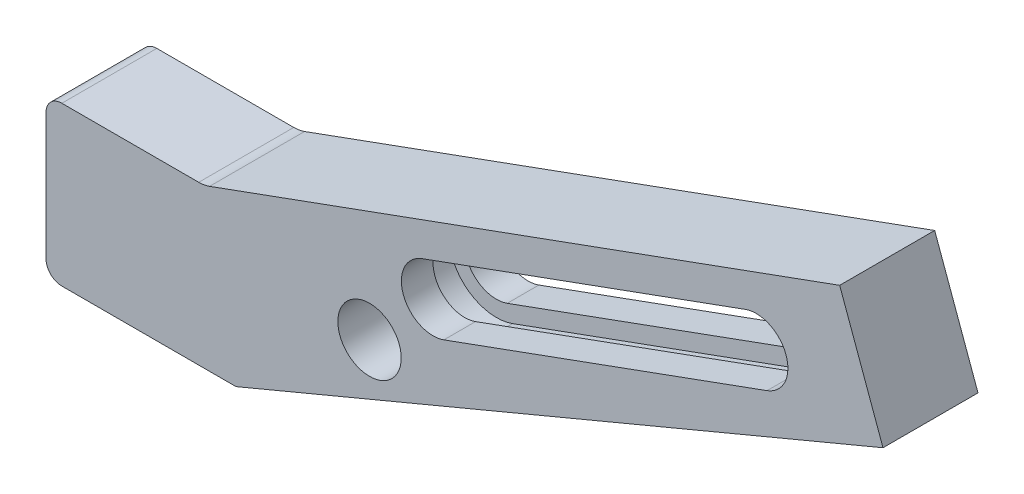
SolidWorks part; units mm, degrees
ref_plane "Front Plane" through (0, 0, 0) normal (0, 0, 1) x (1, 0, 0)
ref_plane "Top Plane" through (0, 0, 0) normal (0, 1, 0) x (1, 0, 0)
ref_plane "Right Plane" through (0, 0, 0) normal (1, 0, 0) x (0, 0, -1)
other "Configuration Table"
sketch "Sketch1" plane through (0, 0, 0) normal (0, 0, 1) x (1, 0, 0)
  line L0 (0, 0) -> (0, 50)
  line L1 (0, 50) -> (50, 50)
  line L2 (50, 50) -> (250.635, 123.0252)
  line L3 (250.635, 123.0252) -> (264.3158, 85.4375)
  line L4 (264.3158, 85.4375) -> (60, 0)
  line L5 (60, 0) -> (0, 0)
  line L6 (122.2292, 55.0057) -> (224.2867, 92.1516) construction
  line L9 (118.809, 64.4026) -> (220.8665, 101.5485)
  line L10 (125.6494, 45.6088) -> (227.7069, 82.7547)
  arc A2 (118.809, 64.4026) -> (125.6494, 45.6088) centre (122.2292, 55.0057) ccw
  arc A3 (227.7069, 82.7547) -> (220.8665, 101.5485) centre (224.2867, 92.1516) ccw
  point P9 (173.2579, 73.5787)
  dimension "D1" = 50
  dimension "D2" = 50
  dimension "D3" = 60
  dimension "D4" = 40
  dimension "D5" = 20
  dimension "D6" = 20
extrude "Boss-Extrude1" add sketch "Sketch1" along normal mid plane 30
fillet "Fillet1" radius 10 1 edges at (50, 50, 0)
fillet "Fillet2" radius 5 2 edges at (0, 0, 0) (0, 50, 0)
ref_plane "Plane1" through (1.1662, 1.6051, 0) normal (-0.5878, -0.809, 0) x (0, 0, -1)
sketch "Sketch2" plane through (1.1662, 1.6051, 0) normal (-0.5878, -0.809, 0) x (0, 0, -1)
  circle A0 centre (0, 0) radius 5
  dimension "D1" = 10
extrude "Cut-Extrude1" cut sketch "Sketch2" against normal blind 10
sketch "Sketch3" plane through (0, 0, 0) normal (-1, 0, 0) x (0, 0, 1)
  line L0 (15, 45) -> (-15, 45) construction
  circle A0 centre (0, 40) radius 5
  dimension "D1" = 10
  dimension "D2" = 5
extrude "Cut-Extrude2" cut sketch "Sketch3" against normal blind 10 contours A0
sketch "Sketch5" plane through (0, 0, -15) normal (0, 0, -1) x (-1, 0, 0)
  line L0 (0, 45) -> (0, 5) construction
  circle A0 centre (-15, 25.1116) radius 10
  dimension "D1" = 20
  dimension "D2" = 15
extrude "Boss-Extrude3" add sketch "Sketch5" along normal blind 10
sketch "Sketch6" plane through (0, 0, -25) normal (0, 0, -1) x (-1, 0, 0)
  circle A0 centre (-15, 25.1116) radius 7.5
  dimension "D1" = 15
extrude "Boss-Extrude4" add sketch "Sketch6" along normal blind 5
sketch "Sketch7" plane through (0, 0, -30) normal (0, 0, -1) x (-1, 0, 0)
  circle A0 centre (-15, 25.1116) radius 10
extrude "Boss-Extrude5" add sketch "Sketch7" along normal blind 2
sketch "Sketch8" plane through (0, 0, 15) normal (0, 0, 1) x (1, 0, 0)
  line L4 (264.3158, 85.4375) -> (250.635, 123.0252) construction
  line L5 (60, 0) -> (264.3158, 85.4375) construction
  circle A0 centre (102.1669, 33.8913) radius 10
  dimension "D1" = 20
  dimension "D2" = 15
  dimension "D3" = 170
extrude "Cut-Extrude3" cut sketch "Sketch8" against normal blind 80
sketch "Sketch9" plane through (0, 0, 0) normal (0, 0, 1) x (1, 0, 0)
  line L1 (220.8665, 101.5485) -> (118.809, 64.4026) construction
  line L2 (220.8665, 101.5485) -> (118.809, 64.4026)
  line L3 (125.6494, 45.6088) -> (227.7069, 82.7547) construction
  line L4 (125.6494, 45.6088) -> (227.7069, 82.7547)
  line L5 (127.3595, 40.9103) -> (229.417, 78.0562)
  line L6 (219.1564, 106.247) -> (117.0989, 69.1011)
  arc A0 (118.809, 64.4026) -> (125.6494, 45.6088) centre (122.2292, 55.0057) ccw construction
  arc A1 (118.809, 64.4026) -> (125.6494, 45.6088) centre (122.2292, 55.0057) ccw
  arc A2 (227.7069, 82.7547) -> (220.8665, 101.5485) centre (224.2867, 92.1516) ccw construction
  arc A3 (227.7069, 82.7547) -> (220.8665, 101.5485) centre (224.2867, 92.1516) ccw
  arc A4 (229.417, 78.0562) -> (219.1564, 106.247) centre (224.2867, 92.1516) ccw
  arc A5 (117.0989, 69.1011) -> (127.3595, 40.9103) centre (122.2292, 55.0057) ccw
  dimension "D1" = 5
extrude "Cut-Extrude4" cut sketch "Sketch9" against normal mid plane 10
sketch "Sketch10" plane through (0, 0, 0) normal (-1, 0, 0) x (0, 0, 1)
  line L1 (-48.0708, 51.4765) -> (-15, 51.4765)
  line L2 (-48.0708, 51.4765) -> (-48.0708, 0)
  line L3 (-48.0708, 0) -> (-15, 0)
  line L4 (-15, 51.4765) -> (-15, 0)
extrude "Cut-Extrude5" cut sketch "Sketch10" against normal blind 50
